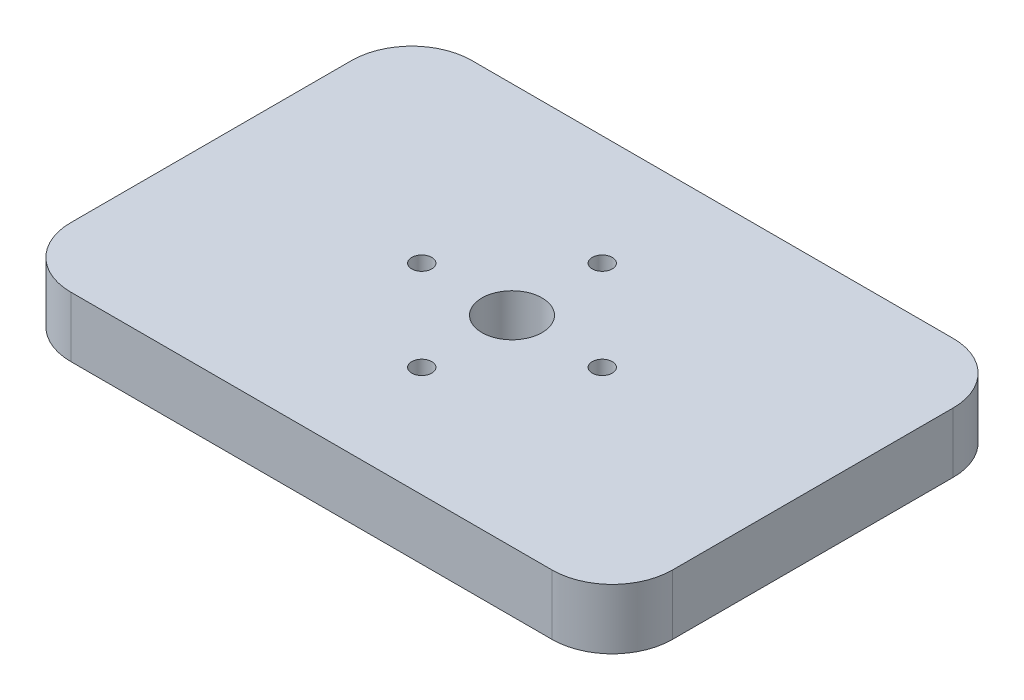
SolidWorks part; units mm, degrees
ref_plane "Front Plane" through (0, 0, 0) normal (0, 0, 1) x (1, 0, 0)
ref_plane "Top Plane" through (0, 0, 0) normal (0, 1, 0) x (1, 0, 0)
ref_plane "Right Plane" through (0, 0, 0) normal (1, 0, 0) x (0, 0, -1)
other "Configuration Table"
sketch "Sketch1" plane through (0, 0, 0) normal (0, 1, 0) x (1, 0, 0)
  line L1 (-150, -100) -> (150, -100)
  line L2 (-150, -100) -> (-150, 100)
  line L3 (-150, 100) -> (150, 100)
  line L4 (150, -100) -> (150, 100)
  line L5 (0, 100) -> (0, -100) construction
  line L6 (-150, 0) -> (150, 0) construction
  point P0 (0, 0)
  dimension "D1" = 200
  dimension "D2" = 300
extrude "Boss-Extrude1" add sketch "Sketch1" along normal blind 30
sketch "Sketch2" plane through (0, 30, 0) normal (0, 1, 0) x (1, 0, 0)
  line L0 (0, 0) -> (0, 50000) construction
  line L1 (0, 0) -> (50000, 0) construction
  circle A0 centre (0, 0) radius 15
  circle A1 centre (0, 0) radius 45 construction
  circle A2 centre (0, 45) radius 5
  circle A3 centre (-45, 0) radius 5
  circle A4 centre (0, -45) radius 5
  circle A5 centre (45, 0) radius 5
  dimension "D1" = 30
  dimension "D2" = 90
  dimension "D3" = 10
extrude "Cut-Extrude1" cut sketch "Sketch2" against normal blind 30
fillet "Fillet1" radius 30 4 edges at (-150, 15, 100) (-150, 15, -100) (150, 15, -100) (150, 15, 100)
